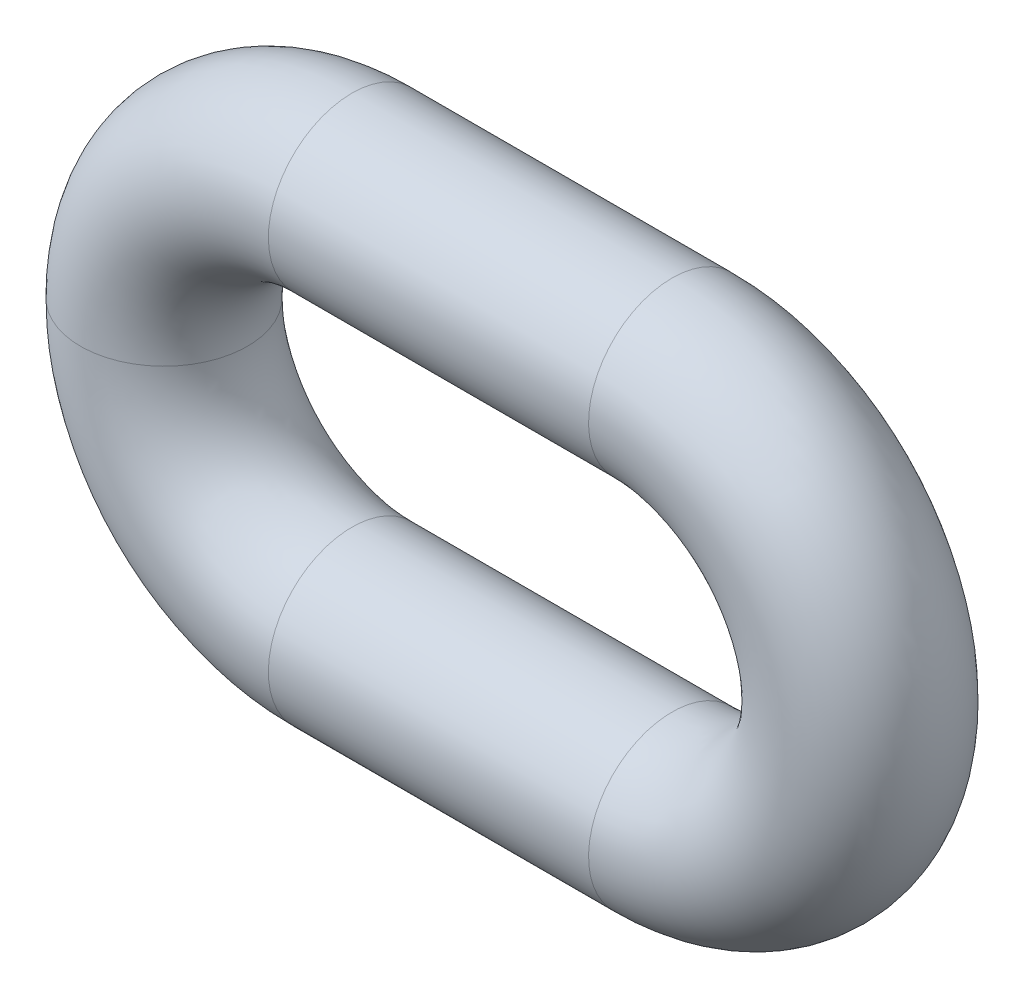
from build123d import *

# Parameters (mm, degrees)
SKETCH_18_R = 24


with BuildPart() as part:
    # 扫描2: sweep along a path in 草图1
    with BuildLine(Plane.XY) as sweep_2_path:
        Line((0, 78), (92, 78))
        ThreePointArc((92, 78), (170, 0), (92, -78))
        Line((92, -78), (0, -78))
        ThreePointArc((0, -78), (-78, 0), (0, 78))
    # 草图18 → 扫描2 (sweep)
    with BuildSketch(Plane(origin=(0, 0, 0), x_dir=(1, 0, 0), z_dir=(0, 1, 0))):
        with Locations((-54, 0)):
            Circle(SKETCH_18_R)
    sweep(path=sweep_2_path.line)


solid = part.part
